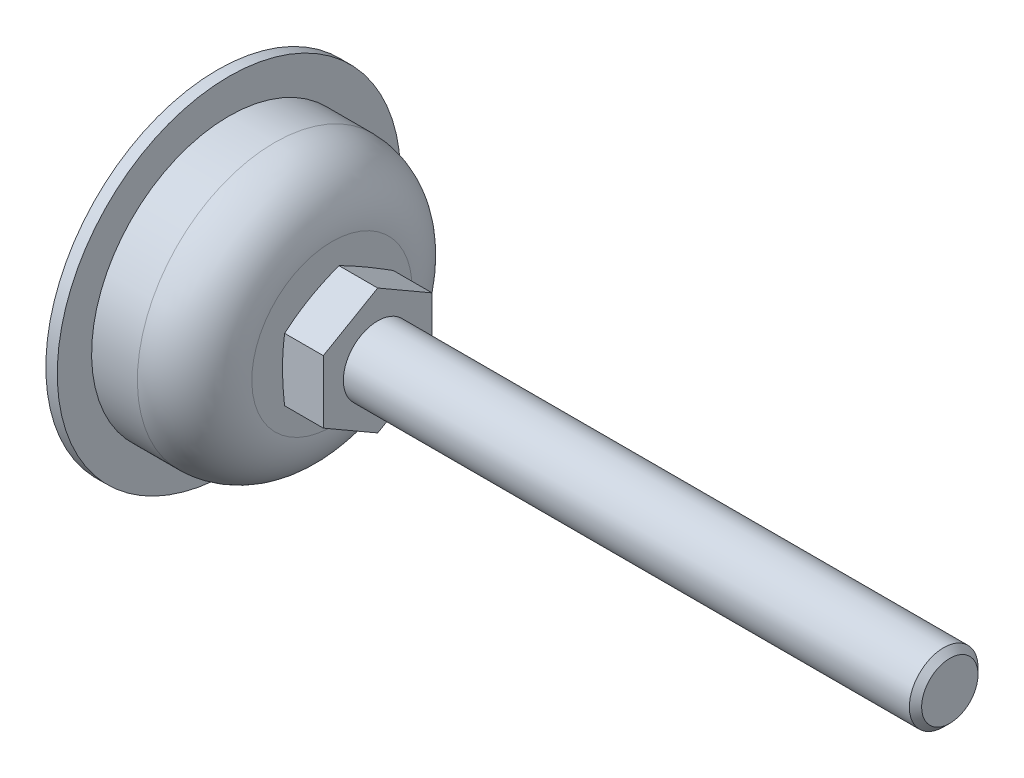
from build123d import *

# Parameters (mm, degrees)
SKETCH_2_R          = 12.35
CUT_EXTRUDE_1_DEPTH = 8


with BuildPart() as part:
    # 草图1 → 旋转1 (revolve)
    with BuildSketch(Plane.XY, mode=Mode.PRIVATE) as revolve_1_sk:
        with BuildLine():
            Line((128, 0), (128, -4.9265))
            Line((128, -4.9265), (126.9265, -6))
            Line((126.9265, -6), (28, -6))
            Line((28, -6), (28, -11.875))
            Line((28, -11.875), (21.461538462, -11.875))
            Line((21.461538462, -11.875), (20, -6))
            Line((20, -6), (20, -14))
            ThreePointArc((20, -14), (17.071067812, -21.071067812), (10, -24))
            Line((10, -24), (2, -24))
            Line((2, -24), (2, -30))
            Line((2, -30), (0, -30))
            Line((0, -30), (0, 0))
            Line((0, 0), (128, 0))
        make_face()
    revolve(revolve_1_sk.sketch.rotate(Axis((0, 0, 0), (1, 0, 0)), 180), axis=Axis((0, 0, 0), (1, 0, 0)))

    # 草图2 → 切除-拉伸1 (cut)
    with BuildSketch(Plane(origin=(28, 0, 0), x_dir=(0, 0, -1), z_dir=(1, 0, 0))):
        Circle(SKETCH_2_R)
        Polygon((-9.5, 5.484827557), (-9.5, -5.484827557), (0, -10.969655115), (9.5, -5.484827557), (9.5, 5.484827557), (0, 10.969655115), align=None, mode=Mode.SUBTRACT)
    extrude(amount=-CUT_EXTRUDE_1_DEPTH, mode=Mode.SUBTRACT)


solid = part.part
